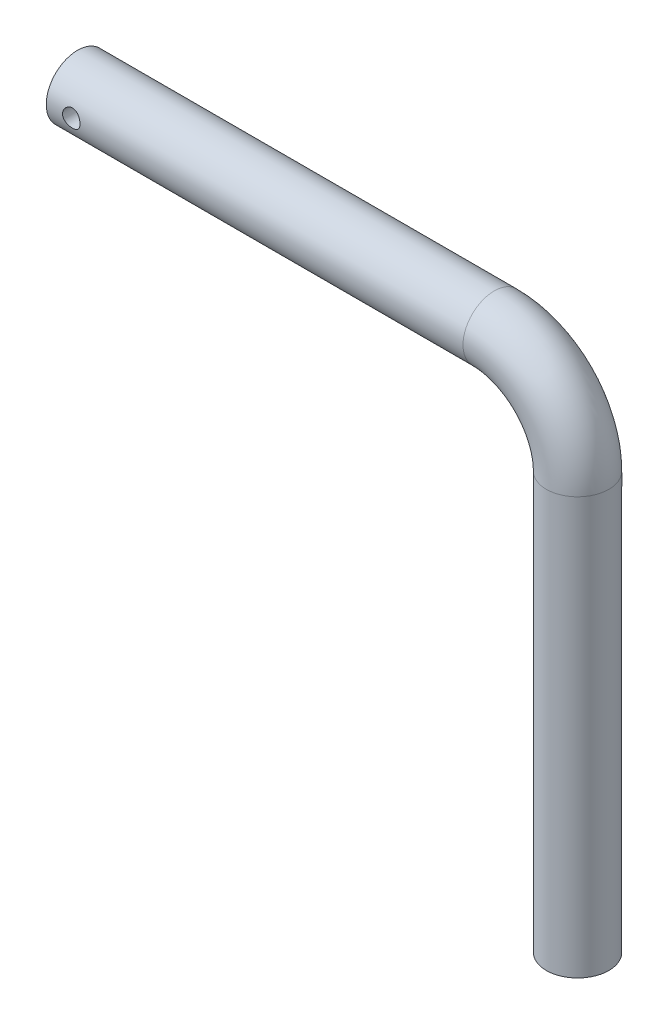
SolidWorks part; units mm, degrees
ref_plane "前视基准面" through (0, 0, 0) normal (0, 0, 1) x (1, 0, 0)
ref_plane "上视基准面" through (0, 0, 0) normal (0, 1, 0) x (1, 0, 0)
ref_plane "右视基准面" through (0, 0, 0) normal (1, 0, 0) x (0, 0, -1)
sketch "草图1" plane through (0, 0, 0) normal (0, 0, 1) x (1, 0, 0)
  line L0 (0, 0) -> (100, 0)
  line L1 (120, -20) -> (120, -120)
  arc A0 (100, 0) -> (120, -20) centre (100, -20) cw
  point P6 (120, 0)
  dimension "D3" = 20
  dimension "D1" = 120
  dimension "D2" = 120
sweep "扫描1" add path "草图1" circular profile diameter 15 parameters "D3"=15
ref_plane "基准面1" through (0, 0, 7.5) normal (0, 0, 1) x (1, 0, 0)
sketch "草图6" plane through (0, 0, 7.5) normal (0, 0, 1) x (1, 0, 0)
  line L0 (0, 7.5) -> (0, -7.5) construction
  circle A0 centre (6, 0) radius 2.1
  dimension "D2" = 4.2
  dimension "D1" = 6
extrude "切除-拉伸1" cut sketch "草图6" against normal blind 20
